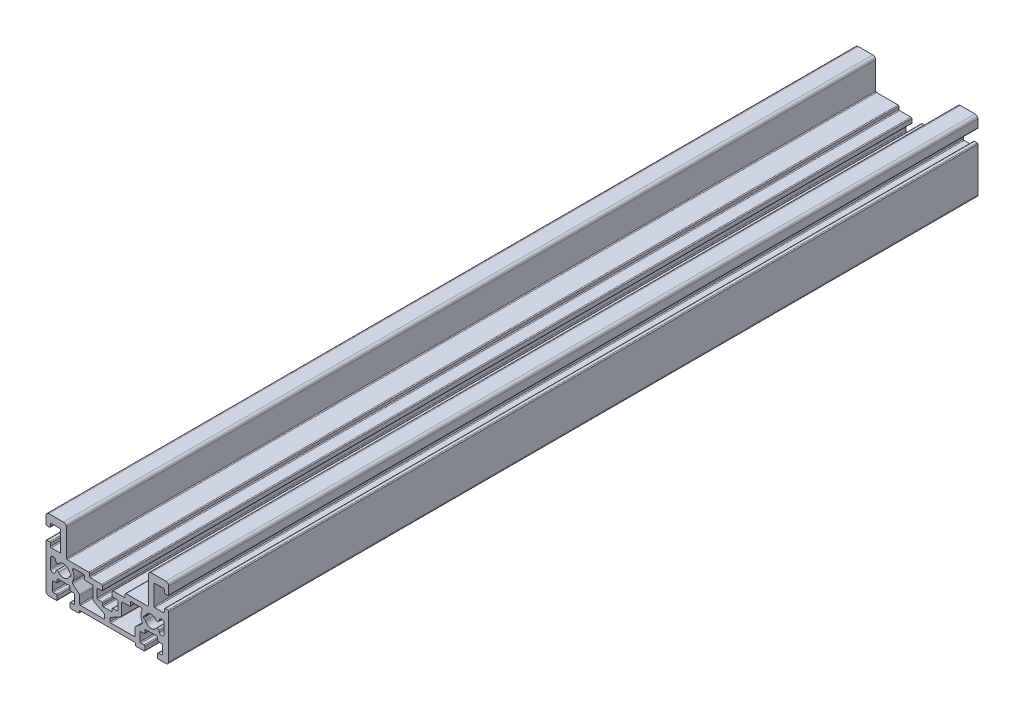
from build123d import *

# Parameters (mm, degrees)
BOSS_EXTRUDE1_DEPTH      = 147
BOSS_EXTRUDE1_DEPTH_BACK = 130


with BuildPart() as part:
    # Sketch3 → Boss-Extrude1 (new, two sides: drawn at the far end of the back side and taken through both)
    with BuildSketch(Plane.XY.offset(-BOSS_EXTRUDE1_DEPTH_BACK)):
        with BuildLine():
            Line((773.343528713, -9082.188023547), (773.343528713, -9079.388023547))
            ThreePointArc((773.343528713, -9079.388023547), (773.431396678, -9079.175891512), (773.643528713, -9079.088023547))
            Line((773.643528713, -9079.088023547), (774.693528713, -9079.088023547))
            ThreePointArc((774.693528713, -9079.088023547), (774.905660747, -9079.000155581), (774.993528713, -9078.788023547))
            Line((774.993528713, -9078.788023547), (774.993528713, -9077.988023547))
            ThreePointArc((774.993528713, -9077.988023547), (775.081396678, -9077.775891512), (775.293528713, -9077.688023547))
            Line((775.293528713, -9077.688023547), (778.993528713, -9077.688023547))
            ThreePointArc((778.993528713, -9077.688023547), (779.205660747, -9077.775891512), (779.293528713, -9077.988023547))
            Line((779.293528713, -9077.988023547), (779.293528713, -9078.788023547))
            ThreePointArc((779.293528713, -9078.788023547), (779.381396678, -9079.000155581), (779.593528713, -9079.088023547))
            Line((779.593528713, -9079.088023547), (780.643528713, -9079.088023547))
            ThreePointArc((780.643528713, -9079.088023547), (780.855660747, -9079.175891512), (780.943528713, -9079.388023547))
            Line((780.943528713, -9079.388023547), (780.943528713, -9082.188023547))
            ThreePointArc((780.943528713, -9082.188023547), (780.855660747, -9082.400155581), (780.643528713, -9082.488023547))
            Line((780.643528713, -9082.488023547), (779.593528713, -9082.488023547))
            ThreePointArc((779.593528713, -9082.488023547), (779.381396678, -9082.575891512), (779.293528713, -9082.788023547))
            Line((779.293528713, -9082.788023547), (779.293528713, -9083.988023547))
            ThreePointArc((779.293528713, -9083.988023547), (779.381396678, -9084.200155581), (779.593528713, -9084.288023547))
            Line((779.593528713, -9084.288023547), (782.243528713, -9084.288023547))
            ThreePointArc((782.243528713, -9084.288023547), (782.455660747, -9084.200155581), (782.543528713, -9083.988023547))
            Line((782.543528713, -9083.988023547), (782.543528713, -9083.588023547))
            ThreePointArc((782.543528713, -9083.588023547), (782.631396678, -9083.375891512), (782.843528713, -9083.288023547))
            Line((782.843528713, -9083.288023547), (801.443528713, -9083.288023547))
            ThreePointArc((801.443528713, -9083.288023547), (801.655660747, -9083.375891512), (801.743528713, -9083.588023547))
            Line((801.743528713, -9083.588023547), (801.743528713, -9083.988023547))
            ThreePointArc((801.743528713, -9083.988023547), (801.831396678, -9084.200155581), (802.043528713, -9084.288023547))
            Line((802.043528713, -9084.288023547), (804.693528713, -9084.288023547))
            ThreePointArc((804.693528713, -9084.288023547), (804.905660747, -9084.200155581), (804.993528713, -9083.988023547))
            Line((804.993528713, -9083.988023547), (804.993528713, -9082.788023547))
            ThreePointArc((804.993528713, -9082.788023547), (804.905660747, -9082.575891512), (804.693528713, -9082.488023547))
            Line((804.693528713, -9082.488023547), (803.643528713, -9082.488023547))
            ThreePointArc((803.643528713, -9082.488023547), (803.431396678, -9082.400155581), (803.343528713, -9082.188023547))
            Line((803.343528713, -9082.188023547), (803.343528713, -9079.388023547))
            ThreePointArc((803.343528713, -9079.388023547), (803.431396678, -9079.175891512), (803.643528713, -9079.088023547))
            Line((803.643528713, -9079.088023547), (804.693528713, -9079.088023547))
            ThreePointArc((804.693528713, -9079.088023547), (804.905660747, -9079.000155581), (804.993528713, -9078.788023547))
            Line((804.993528713, -9078.788023547), (804.993528713, -9077.988023547))
            ThreePointArc((804.993528713, -9077.988023547), (805.081396678, -9077.775891512), (805.293528713, -9077.688023547))
            Line((805.293528713, -9077.688023547), (808.993528713, -9077.688023547))
            ThreePointArc((808.993528713, -9077.688023547), (809.205660747, -9077.775891512), (809.293528713, -9077.988023547))
            Line((809.293528713, -9077.988023547), (809.293528713, -9078.788023547))
            ThreePointArc((809.293528713, -9078.788023547), (809.381396678, -9079.000155581), (809.593528713, -9079.088023547))
            Line((809.593528713, -9079.088023547), (810.643528713, -9079.088023547))
            ThreePointArc((810.643528713, -9079.088023547), (810.855660747, -9079.175891512), (810.943528713, -9079.388023547))
            Line((810.943528713, -9079.388023547), (810.943528713, -9082.188023547))
            ThreePointArc((810.943528713, -9082.188023547), (810.855660747, -9082.400155581), (810.643528713, -9082.488023547))
            Line((810.643528713, -9082.488023547), (809.593528713, -9082.488023547))
            ThreePointArc((809.593528713, -9082.488023547), (809.381396678, -9082.575891512), (809.293528713, -9082.788023547))
            Line((809.293528713, -9082.788023547), (809.293528713, -9083.988023547))
            ThreePointArc((809.293528713, -9083.988023547), (809.381396678, -9084.200155581), (809.593528713, -9084.288023547))
            Line((809.593528713, -9084.288023547), (812.143528713, -9084.288023547))
            ThreePointArc((812.143528713, -9084.288023547), (812.850635494, -9083.995130328), (813.143528713, -9083.288023547))
            Line((813.143528713, -9083.288023547), (813.143528713, -9068.388023547))
            ThreePointArc((813.143528713, -9068.388023547), (813.055660747, -9068.175891512), (812.843528713, -9068.088023547))
            Line((812.843528713, -9068.088023547), (811.943528713, -9068.088023547))
            ThreePointArc((811.943528713, -9068.088023547), (811.731396678, -9068.175891512), (811.643528713, -9068.388023547))
            Line((811.643528713, -9068.388023547), (811.643528713, -9069.288023547))
            ThreePointArc((811.643528713, -9069.288023547), (811.555660747, -9069.500155581), (811.343528713, -9069.588023547))
            Line((811.343528713, -9069.588023547), (808.443528713, -9069.588023547))
            ThreePointArc((808.443528713, -9069.588023547), (808.231396678, -9069.500155581), (808.143528713, -9069.288023547))
            Line((808.143528713, -9069.288023547), (808.143528713, -9062.688023547))
            ThreePointArc((808.143528713, -9062.688023547), (808.231396678, -9062.475891512), (808.443528713, -9062.388023547))
            Line((808.443528713, -9062.388023547), (811.343528713, -9062.388023547))
            ThreePointArc((811.343528713, -9062.388023547), (811.555660747, -9062.475891512), (811.643528713, -9062.688023547))
            Line((811.643528713, -9062.688023547), (811.643528713, -9063.488023547))
            ThreePointArc((811.643528713, -9063.488023547), (811.731396678, -9063.700155581), (811.943528713, -9063.788023547))
            Line((811.943528713, -9063.788023547), (812.843528713, -9063.788023547))
            ThreePointArc((812.843528713, -9063.788023547), (813.055660747, -9063.700155581), (813.143528713, -9063.488023547))
            Line((813.143528713, -9063.488023547), (813.143528713, -9060.888023547))
            ThreePointArc((813.143528713, -9060.888023547), (812.850635494, -9060.180916766), (812.143528713, -9059.888023547))
            Line((812.143528713, -9059.888023547), (807.143528713, -9059.888023547))
            ThreePointArc((807.143528713, -9059.888023547), (806.436421931, -9060.180916766), (806.143528713, -9060.888023547))
            Line((806.143528713, -9060.888023547), (806.143528713, -9070.088023547))
            ThreePointArc((806.143528713, -9070.088023547), (806.055660747, -9070.300155581), (805.843528713, -9070.388023547))
            Line((805.843528713, -9070.388023547), (798.543528713, -9070.388023547))
            ThreePointArc((798.543528713, -9070.388023547), (798.331396678, -9070.475891512), (798.243528713, -9070.688023547))
            Line((798.243528713, -9070.688023547), (798.243528713, -9071.488023547))
            ThreePointArc((798.243528713, -9071.488023547), (798.155660747, -9071.700155581), (797.943528713, -9071.788023547))
            Line((797.943528713, -9071.788023547), (794.093528713, -9071.788023547))
            ThreePointArc((794.093528713, -9071.788023547), (793.881396678, -9071.875891512), (793.793528713, -9072.088023547))
            Line((793.793528713, -9072.088023547), (793.793528713, -9073.388023547))
            ThreePointArc((793.793528713, -9073.388023547), (793.881396678, -9073.600155581), (794.093528713, -9073.688023547))
            Line((794.093528713, -9073.688023547), (795.443528713, -9073.688023547))
            ThreePointArc((795.443528713, -9073.688023547), (795.655660747, -9073.775891512), (795.743528713, -9073.988023547))
            Line((795.743528713, -9073.988023547), (795.743528713, -9076.688023547))
            ThreePointArc((795.743528713, -9076.688023547), (795.655660747, -9076.900155581), (795.443528713, -9076.988023547))
            Line((795.443528713, -9076.988023547), (794.093528713, -9076.988023547))
            ThreePointArc((794.093528713, -9076.988023547), (793.881396678, -9077.075891512), (793.793528713, -9077.288023547))
            Line((793.793528713, -9077.288023547), (793.793528713, -9077.888023547))
            ThreePointArc((793.793528713, -9077.888023547), (793.705660747, -9078.100155581), (793.493528713, -9078.188023547))
            Line((793.493528713, -9078.188023547), (790.793528713, -9078.188023547))
            ThreePointArc((790.793528713, -9078.188023547), (790.581396678, -9078.100155581), (790.493528713, -9077.888023547))
            Line((790.493528713, -9077.888023547), (790.493528713, -9077.288023547))
            ThreePointArc((790.493528713, -9077.288023547), (790.405660747, -9077.075891512), (790.193528713, -9076.988023547))
            Line((790.193528713, -9076.988023547), (788.843528713, -9076.988023547))
            ThreePointArc((788.843528713, -9076.988023547), (788.631396678, -9076.900155581), (788.543528713, -9076.688023547))
            Line((788.543528713, -9076.688023547), (788.543528713, -9073.988023547))
            ThreePointArc((788.543528713, -9073.988023547), (788.631396678, -9073.775891512), (788.843528713, -9073.688023547))
            Line((788.843528713, -9073.688023547), (790.193528713, -9073.688023547))
            ThreePointArc((790.193528713, -9073.688023547), (790.405660747, -9073.600155581), (790.493528713, -9073.388023547))
            Line((790.493528713, -9073.388023547), (790.493528713, -9072.088023547))
            ThreePointArc((790.493528713, -9072.088023547), (790.405660747, -9071.875891512), (790.193528713, -9071.788023547))
            Line((790.193528713, -9071.788023547), (786.343528713, -9071.788023547))
            ThreePointArc((786.343528713, -9071.788023547), (786.131396678, -9071.700155581), (786.043528713, -9071.488023547))
            Line((786.043528713, -9071.488023547), (786.043528713, -9070.688023547))
            ThreePointArc((786.043528713, -9070.688023547), (785.955660747, -9070.475891512), (785.743528713, -9070.388023547))
            Line((785.743528713, -9070.388023547), (778.443528713, -9070.388023547))
            ThreePointArc((778.443528713, -9070.388023547), (778.231396678, -9070.300155581), (778.143528713, -9070.088023547))
            Line((778.143528713, -9070.088023547), (778.143528713, -9060.888023547))
            ThreePointArc((778.143528713, -9060.888023547), (777.850635494, -9060.180916766), (777.143528713, -9059.888023547))
            Line((777.143528713, -9059.888023547), (772.143528713, -9059.888023547))
            ThreePointArc((772.143528713, -9059.888023547), (771.436421931, -9060.180916766), (771.143528713, -9060.888023547))
            Line((771.143528713, -9060.888023547), (771.143528713, -9063.488023547))
            ThreePointArc((771.143528713, -9063.488023547), (771.231396678, -9063.700155581), (771.443528713, -9063.788023547))
            Line((771.443528713, -9063.788023547), (772.343528713, -9063.788023547))
            ThreePointArc((772.343528713, -9063.788023547), (772.555660747, -9063.700155581), (772.643528713, -9063.488023547))
            Line((772.643528713, -9063.488023547), (772.643528713, -9062.688023547))
            ThreePointArc((772.643528713, -9062.688023547), (772.731396678, -9062.475891512), (772.943528713, -9062.388023547))
            Line((772.943528713, -9062.388023547), (775.843528713, -9062.388023547))
            ThreePointArc((775.843528713, -9062.388023547), (776.055660747, -9062.475891512), (776.143528713, -9062.688023547))
            Line((776.143528713, -9062.688023547), (776.143528713, -9069.288023547))
            ThreePointArc((776.143528713, -9069.288023547), (776.055660747, -9069.500155581), (775.843528713, -9069.588023547))
            Line((775.843528713, -9069.588023547), (772.943528713, -9069.588023547))
            ThreePointArc((772.943528713, -9069.588023547), (772.731396678, -9069.500155581), (772.643528713, -9069.288023547))
            Line((772.643528713, -9069.288023547), (772.643528713, -9068.388023547))
            ThreePointArc((772.643528713, -9068.388023547), (772.555660747, -9068.175891512), (772.343528713, -9068.088023547))
            Line((772.343528713, -9068.088023547), (771.443528713, -9068.088023547))
            ThreePointArc((771.443528713, -9068.088023547), (771.231396678, -9068.175891512), (771.143528713, -9068.388023547))
            Line((771.143528713, -9068.388023547), (771.143528713, -9083.288023547))
            ThreePointArc((771.143528713, -9083.288023547), (771.436421931, -9083.995130328), (772.143528713, -9084.288023547))
            Line((772.143528713, -9084.288023547), (774.693528713, -9084.288023547))
            ThreePointArc((774.693528713, -9084.288023547), (774.905660747, -9084.200155581), (774.993528713, -9083.988023547))
            Line((774.993528713, -9083.988023547), (774.993528713, -9082.788023547))
            ThreePointArc((774.993528713, -9082.788023547), (774.905660747, -9082.575891512), (774.693528713, -9082.488023547))
            Line((774.693528713, -9082.488023547), (773.643528713, -9082.488023547))
            ThreePointArc((773.643528713, -9082.488023547), (773.431396678, -9082.400155581), (773.343528713, -9082.188023547))
        make_face()
        with BuildLine():
            Line((780.753297488, -9071.888023547), (783.943528713, -9071.888023547))
            ThreePointArc((783.943528713, -9071.888023547), (784.155660747, -9071.975891512), (784.243528713, -9072.188023547))
            Line((784.243528713, -9072.188023547), (784.243528713, -9073.188023547))
            ThreePointArc((784.243528713, -9073.188023547), (784.331396678, -9073.400155581), (784.543528713, -9073.488023547))
            Line((784.543528713, -9073.488023547), (786.943528713, -9073.488023547))
            ThreePointArc((786.943528713, -9073.488023547), (787.155660747, -9073.575891512), (787.243528713, -9073.788023547))
            Line((787.243528713, -9073.788023547), (787.243528713, -9077.81064218))
            ThreePointArc((787.243528713, -9077.81064218), (787.285291721, -9077.963330282), (787.398953088, -9078.073506953))
            Line((787.398953088, -9078.073506953), (791.088104337, -9080.10254014))
            ThreePointArc((791.088104337, -9080.10254014), (791.201765704, -9080.212716812), (791.243528713, -9080.365404913))
            Line((791.243528713, -9080.365404913), (791.243528713, -9081.388023547))
            ThreePointArc((791.243528713, -9081.388023547), (791.155660747, -9081.600155581), (790.943528713, -9081.688023547))
            Line((790.943528713, -9081.688023547), (782.993528713, -9081.688023547))
            ThreePointArc((782.993528713, -9081.688023547), (782.781396678, -9081.600155581), (782.693528713, -9081.388023547))
            Line((782.693528713, -9081.388023547), (782.693528713, -9078.916705878))
            ThreePointArc((782.693528713, -9078.916705878), (782.648227807, -9078.70874258), (782.52053378, -9078.538462985))
            Line((782.52053378, -9078.538462985), (780.288753954, -9076.60900621))
            ThreePointArc((780.288753954, -9076.60900621), (780.121624324, -9076.307123653), (780.189832059, -9075.968873604))
            ThreePointArc((780.189832059, -9075.968873604), (780.691353015, -9074.309637702), (780.309737388, -9072.618792778))
            ThreePointArc((780.309737388, -9072.618792778), (780.325872281, -9072.128586286), (780.753297488, -9071.888023547))
        make_face(mode=Mode.SUBTRACT)
        with BuildLine():
            Line((772.693528713, -9075.878570126), (772.693528713, -9072.697476968))
            ThreePointArc((772.693528713, -9072.697476968), (773.403410955, -9071.851138593), (774.360375636, -9072.402899449))
            ThreePointArc((774.360375636, -9072.402899449), (774.444451093, -9072.651620738), (774.516561223, -9072.904070913))
            ThreePointArc((774.516561223, -9072.904070913), (774.920449025, -9073.279587676), (775.431394634, -9073.072047849))
            ThreePointArc((775.431394634, -9073.072047849), (777.434187003, -9072.208235636), (779.1234277, -9073.588023547))
            ThreePointArc((779.1234277, -9073.588023547), (779.233065331, -9073.732972522), (779.406270411, -9073.788023547))
            Line((779.406270411, -9073.788023547), (779.393528714, -9073.788023547))
            ThreePointArc((779.393528714, -9073.788023547), (779.605660748, -9073.875891513), (779.693528714, -9074.088023547))
            Line((779.693528714, -9074.088023547), (779.693528714, -9074.488023547))
            ThreePointArc((779.693528714, -9074.488023547), (779.605660748, -9074.700155582), (779.393528714, -9074.788023547))
            Line((779.393528714, -9074.788023547), (779.406270411, -9074.788023547))
            ThreePointArc((779.406270411, -9074.788023547), (779.233065331, -9074.843074573), (779.123427699, -9074.988023547))
            ThreePointArc((779.123427699, -9074.988023547), (777.434187002, -9076.367811459), (775.431394634, -9075.503999244))
            ThreePointArc((775.431394634, -9075.503999244), (774.920449025, -9075.296459417), (774.516561223, -9075.67197618))
            ThreePointArc((774.516561223, -9075.67197618), (774.444451093, -9075.924426356), (774.360375636, -9076.173147645))
            ThreePointArc((774.360375636, -9076.173147645), (773.403410955, -9076.724908501), (772.693528713, -9075.878570126))
        make_face(mode=Mode.SUBTRACT)
        with BuildLine():
            Line((803.998303472, -9076.60900621), (801.766523645, -9078.538462985))
            ThreePointArc((801.766523645, -9078.538462985), (801.638829618, -9078.70874258), (801.593528713, -9078.916705878))
            Line((801.593528713, -9078.916705878), (801.593528713, -9081.388023547))
            ThreePointArc((801.593528713, -9081.388023547), (801.505660747, -9081.600155581), (801.293528713, -9081.688023547))
            Line((801.293528713, -9081.688023547), (793.343528713, -9081.688023547))
            ThreePointArc((793.343528713, -9081.688023547), (793.131396678, -9081.600155581), (793.043528713, -9081.388023547))
            Line((793.043528713, -9081.388023547), (793.043528713, -9080.365404913))
            ThreePointArc((793.043528713, -9080.365404913), (793.085291721, -9080.212716812), (793.198953088, -9080.10254014))
            Line((793.198953088, -9080.10254014), (796.888104337, -9078.073506953))
            ThreePointArc((796.888104337, -9078.073506953), (797.001765704, -9077.963330282), (797.043528713, -9077.81064218))
            Line((797.043528713, -9077.81064218), (797.043528713, -9073.788023547))
            ThreePointArc((797.043528713, -9073.788023547), (797.131396678, -9073.575891512), (797.343528713, -9073.488023547))
            Line((797.343528713, -9073.488023547), (799.743528713, -9073.488023547))
            ThreePointArc((799.743528713, -9073.488023547), (799.955660747, -9073.400155581), (800.043528713, -9073.188023547))
            Line((800.043528713, -9073.188023547), (800.043528713, -9072.188023547))
            ThreePointArc((800.043528713, -9072.188023547), (800.131396678, -9071.975891512), (800.343528713, -9071.888023547))
            Line((800.343528713, -9071.888023547), (803.533759937, -9071.888023547))
            ThreePointArc((803.533759937, -9071.888023547), (803.961185144, -9072.128586286), (803.977320037, -9072.618792778))
            ThreePointArc((803.977320037, -9072.618792778), (803.59570441, -9074.309637702), (804.097225367, -9075.968873603))
            ThreePointArc((804.097225367, -9075.968873603), (804.165433102, -9076.307123653), (803.998303472, -9076.60900621))
        make_face(mode=Mode.SUBTRACT)
        with BuildLine():
            Line((804.880787015, -9074.788023547), (804.893528713, -9074.788023547))
            ThreePointArc((804.893528713, -9074.788023547), (804.681396678, -9074.700155581), (804.593528713, -9074.488023547))
            Line((804.593528713, -9074.488023547), (804.593528713, -9074.088023547))
            ThreePointArc((804.593528713, -9074.088023547), (804.681396678, -9073.875891512), (804.893528713, -9073.788023547))
            Line((804.893528713, -9073.788023547), (804.880787015, -9073.788023547))
            ThreePointArc((804.880787015, -9073.788023547), (805.053992095, -9073.73297252), (805.163629725, -9073.588023546))
            ThreePointArc((805.163629725, -9073.588023546), (806.852870423, -9072.208235634), (808.855662793, -9073.072047848))
            ThreePointArc((808.855662793, -9073.072047848), (809.366608402, -9073.279587675), (809.770496204, -9072.904070913))
            ThreePointArc((809.770496204, -9072.904070913), (809.842606334, -9072.651620737), (809.92668179, -9072.402899448))
            ThreePointArc((809.92668179, -9072.402899448), (810.88364647, -9071.851138596), (811.593528713, -9072.697476967))
            Line((811.593528713, -9072.697476967), (811.593528713, -9075.878570125))
            ThreePointArc((811.593528713, -9075.878570125), (810.88364647, -9076.7249085), (809.926681789, -9076.173147644))
            ThreePointArc((809.926681789, -9076.173147644), (809.842606332, -9075.924426355), (809.770496202, -9075.671976179))
            ThreePointArc((809.770496202, -9075.671976179), (809.3666084, -9075.296459417), (808.855662791, -9075.503999244))
            ThreePointArc((808.855662791, -9075.503999244), (806.852870424, -9076.367811457), (805.163629727, -9074.988023547))
            ThreePointArc((805.163629727, -9074.988023547), (805.053992096, -9074.843074572), (804.880787015, -9074.788023547))
        make_face(mode=Mode.SUBTRACT)
    extrude(amount=BOSS_EXTRUDE1_DEPTH + BOSS_EXTRUDE1_DEPTH_BACK)


solid = part.part
